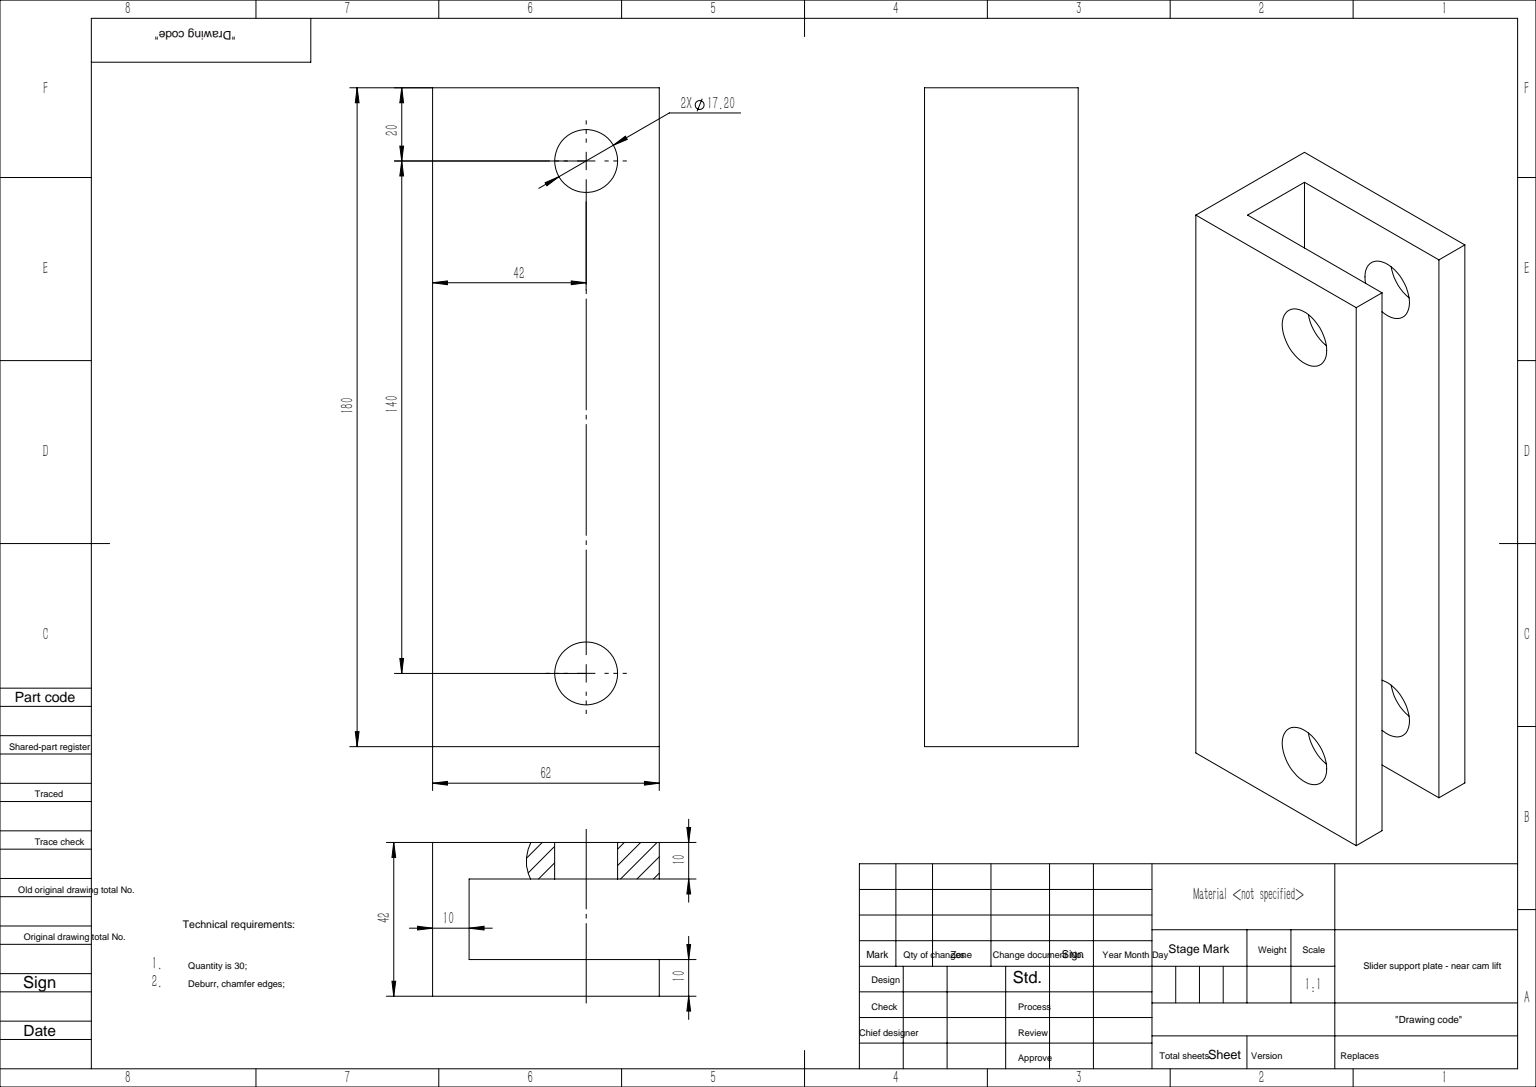
from build123d import *

# Parameters (mm, degrees)
EXTRUDE_1_DEPTH     = 180
SKETCH_2_R          = 8.6
CUT_EXTRUDE_1_DEPTH = 195.956405383


with BuildPart() as part:
    # 草图1 → 凸台-拉伸1 (new body)
    with BuildSketch(Plane(origin=(0, 0, 0), x_dir=(1, 0, 0), z_dir=(0, 1, 0))):
        Polygon((62, 11), (10, 11), (10, -11), (62, -11), (62, -21), (0, -21), (0, 21), (62, 21), align=None)
    extrude(amount=EXTRUDE_1_DEPTH)

    # 草图2 → 切除-拉伸1 (cut, through all)
    with BuildSketch(Plane.XY.offset(21)):
        with Locations((42, 160)):
            Circle(SKETCH_2_R)
        with Locations((42, 20)):
            Circle(SKETCH_2_R)
    extrude(amount=-CUT_EXTRUDE_1_DEPTH, mode=Mode.SUBTRACT)


solid = part.part
